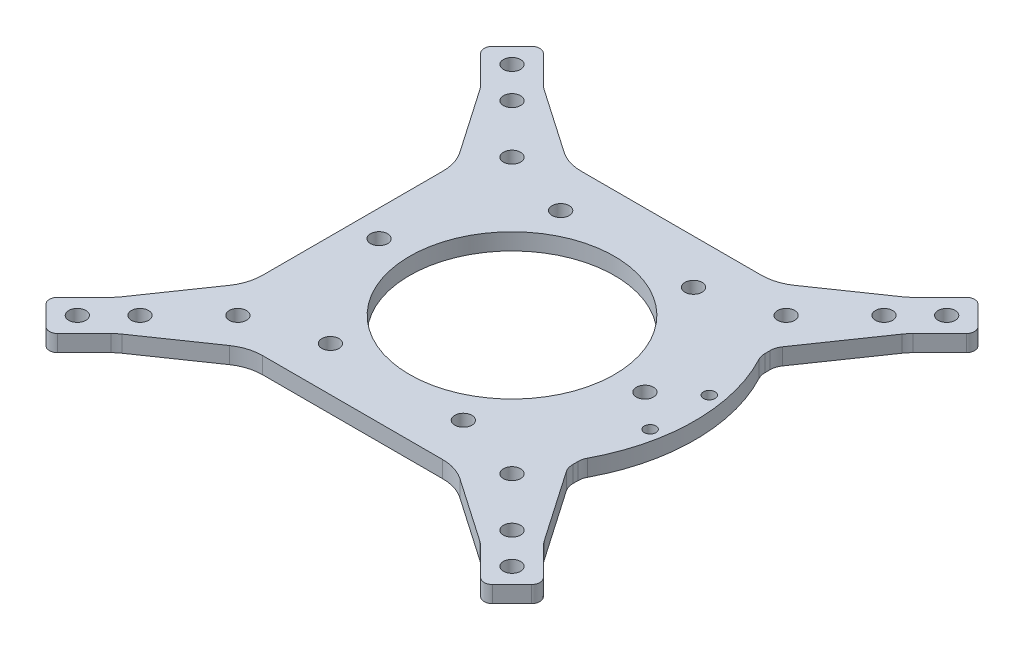
from build123d import *

# Parameters (mm, degrees)
SKETCH_1_R      = 1.55
SKETCH_1_R_2    = 18.5
EXTRUDE_1_DEPTH = 3
SKETCH_2_R      = 1.05
EXTRUDE_2_DEPTH = 3
FILLET_1_R      = 1.5
FILLET_2_R      = 8
FILLET_3_R      = 3


with BuildPart() as part:
    # 草图1 → 凸台-拉伸1 (new body)
    with BuildSketch(Plane(origin=(0, 0, 0), x_dir=(1, 0, 0), z_dir=(0, 1, 0))):
        Polygon((44.901280605, 39.244426356), (39.244426356, 44.901280605), (32.880465325, 38.537319575), (18.748737342, 28.798737342), (-18.748737342, 28.798737342), (-32.880465325, 38.537319575), (-39.244426356, 44.901280605), (-44.901280605, 39.244426356), (-38.537319575, 32.880465325), (-28.798737342, 18.748737342), (-28.798737342, -18.748737342), (-38.537319575, -32.880465325), (-44.901280605, -39.244426356), (-39.244426356, -44.901280605), (-32.880465325, -38.537319575), (-18.748737342, -28.798737342), (18.748737342, -28.798737342), (32.880465325, -38.537319575), (39.244426356, -44.901280605), (44.901280605, -39.244426356), (38.537319575, -32.880465325), (28.798737342, -18.748737342), (28.798737342, 18.748737342), (38.537319575, 32.880465325), align=None)
        with Locations(Location((-39.244426356, -39.244426356, 0), (0, 0, 270))):
            Circle(SKETCH_1_R, mode=Mode.SUBTRACT)
        with Locations(Location((-33.587572106, -33.587572106, 0), (0, 0, 270))):
            Circle(SKETCH_1_R, mode=Mode.SUBTRACT)
        with Locations(Location((-24.748737342, -24.748737342, 0), (0, 0, 270))):
            Circle(SKETCH_1_R, mode=Mode.SUBTRACT)
        with Locations(Location((-12, -20.784609691, 0), (0, 0, 270))):
            Circle(SKETCH_1_R, mode=Mode.SUBTRACT)
        with Locations(Location((39.244426356, -39.244426356, 0), (0, 0, 270))):
            Circle(SKETCH_1_R, mode=Mode.SUBTRACT)
        with Locations(Location((33.587572106, -33.587572106, 0), (0, 0, 270))):
            Circle(SKETCH_1_R, mode=Mode.SUBTRACT)
        with Locations(Location((24.748737342, -24.748737342, 0), (0, 0, 270))):
            Circle(SKETCH_1_R, mode=Mode.SUBTRACT)
        with Locations(Location((12, -20.784609691, 0), (0, 0, 270))):
            Circle(SKETCH_1_R, mode=Mode.SUBTRACT)
        with Locations(Location((-24, 0, 0), (0, 0, 270))):
            Circle(SKETCH_1_R, mode=Mode.SUBTRACT)
        with Locations(Location((-12, 20.784609691, 0), (0, 0, 270))):
            Circle(SKETCH_1_R, mode=Mode.SUBTRACT)
        with Locations(Location((-24.748737342, 24.748737342, 0), (0, 0, 270))):
            Circle(SKETCH_1_R, mode=Mode.SUBTRACT)
        with Locations(Location((-33.587572106, 33.587572106, 0), (0, 0, 270))):
            Circle(SKETCH_1_R, mode=Mode.SUBTRACT)
        with Locations(Location((-39.244426356, 39.244426356, 0), (0, 0, 270))):
            Circle(SKETCH_1_R, mode=Mode.SUBTRACT)
        with Locations(Location((0, 0, 0), (0, 0, 270))):
            Circle(SKETCH_1_R_2, mode=Mode.SUBTRACT)
        with Locations(Location((12, 20.784609691, 0), (0, 0, 270))):
            Circle(SKETCH_1_R, mode=Mode.SUBTRACT)
        with Locations(Location((24, 0, 0), (0, 0, 270))):
            Circle(SKETCH_1_R, mode=Mode.SUBTRACT)
        with Locations(Location((24.748737342, 24.748737342, 0), (0, 0, 270))):
            Circle(SKETCH_1_R, mode=Mode.SUBTRACT)
        with Locations(Location((33.587572106, 33.587572106, 0), (0, 0, 270))):
            Circle(SKETCH_1_R, mode=Mode.SUBTRACT)
        with Locations(Location((39.244426356, 39.244426356, 0), (0, 0, 270))):
            Circle(SKETCH_1_R, mode=Mode.SUBTRACT)
    extrude(amount=EXTRUDE_1_DEPTH)

    # 草图2 → 凸台-拉伸2 (add)
    with BuildSketch(Plane(origin=(0, 3, 0), x_dir=(1, 0, 0), z_dir=(0, 1, 0))):
        with BuildLine():
            Line((28.798737342, 16.113122836), (28.798737342, -16.113122836))
            ThreePointArc((28.798737342, -16.113122836), (33, 0), (28.798737342, 16.113122836))
        make_face()
        with Locations(Location((30.282838405, 5.339681463, 0), (0, 0, 270))):
            Circle(SKETCH_2_R, mode=Mode.SUBTRACT)
        with Locations(Location((30.282838405, -5.339681463, 0), (0, 0, 270))):
            Circle(SKETCH_2_R, mode=Mode.SUBTRACT)
    extrude(amount=-EXTRUDE_2_DEPTH)

    # 圆角1
    fillet_1_edges = [part.edges().sort_by_distance(p)[0] for p in [
        (39.244426356, 1.5, -44.901280605),
        (44.901280605, 1.5, -39.244426356),
        (44.901280605, 1.5, 39.244426356),
        (39.244426356, 1.5, 44.901280605),
        (-39.244426356, 1.5, 44.901280605),
        (-44.901280605, 1.5, 39.244426356),
        (-44.901280605, 1.5, -39.244426356),
        (-39.244426356, 1.5, -44.901280605),
    ]]
    fillet(fillet_1_edges, radius=FILLET_1_R)

    # 圆角2
    fillet_2_edges = [part.edges().sort_by_distance(p)[0] for p in [
        (18.748737342, 1.5, -28.798737342),
        (32.880465325, 1.5, -38.537319575),
        (38.537319575, 1.5, -32.880465325),
        (38.537319575, 1.5, 32.880465325),
        (32.880465325, 1.5, 38.537319575),
        (18.748737342, 1.5, 28.798737342),
        (-18.748737342, 1.5, 28.798737342),
        (-32.880465325, 1.5, 38.537319575),
        (-38.537319575, 1.5, 32.880465325),
        (-28.798737342, 1.5, 18.748737342),
        (-28.798737342, 1.5, -18.748737342),
        (-38.537319575, 1.5, -32.880465325),
        (-32.880465325, 1.5, -38.537319575),
        (-18.748737342, 1.5, -28.798737342),
    ]]
    fillet(fillet_2_edges, radius=FILLET_2_R)

    # 圆角3
    fillet_3_edges = [part.edges().sort_by_distance(p)[0] for p in [
        (28.798737342, 1.5, 16.113122836),
        (28.798737342, 1.5, -16.113122836),
        (28.798737342, 1.5, -18.748737342),
        (28.798737342, 1.5, 18.748737342),
    ]]
    fillet(fillet_3_edges, radius=FILLET_3_R)


solid = part.part
